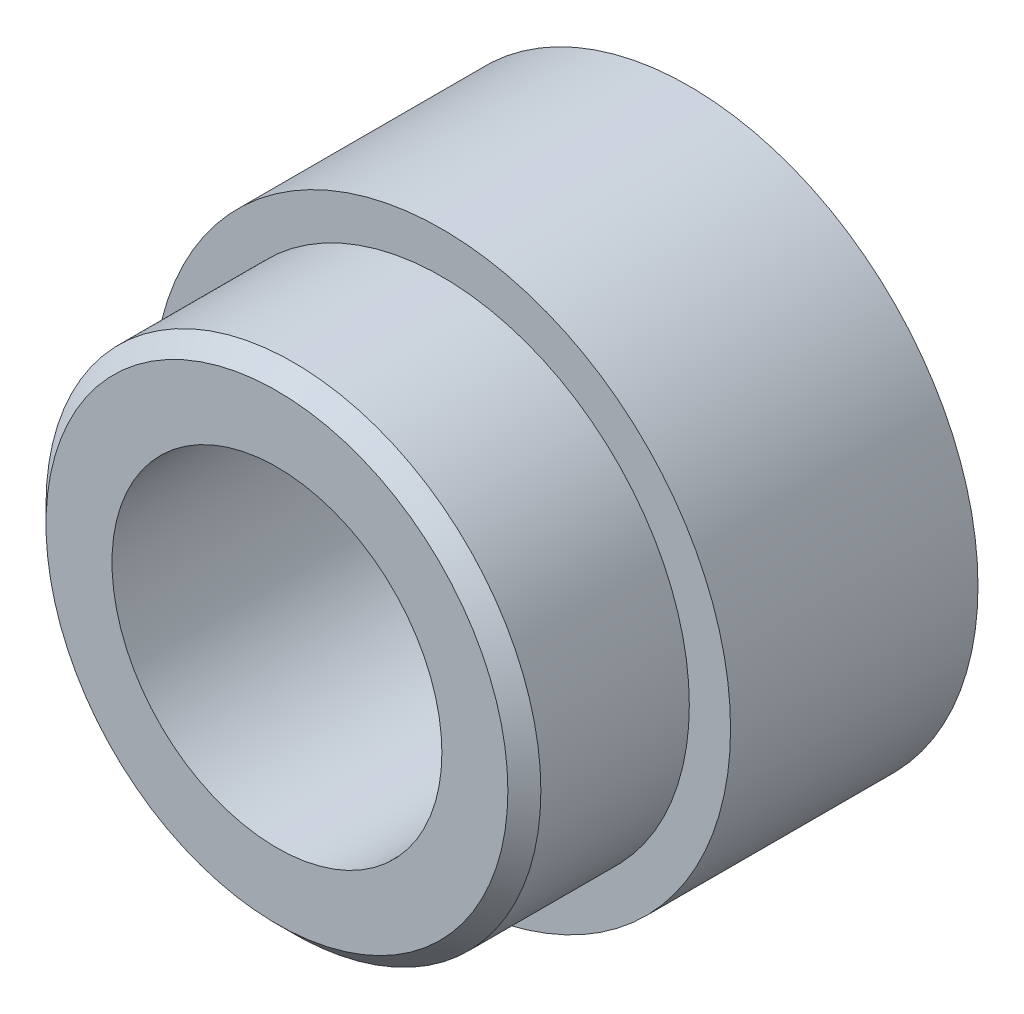
from build123d import *

# Parameters (mm, degrees)
SKETCH1_R           = 17.5
SKETCH1_R_2         = 10
BOSS_EXTRUDE1_DEPTH = 25
CUT_EXTRUDE1_START  = -10
SKETCH2_R           = 17.5
SKETCH2_R_2         = 15
CUT_EXTRUDE1_DEPTH  = 10
CHAMFER1_SIZE       = 1


with BuildPart() as part:
    # Sketch1 → Boss-Extrude1 (new body)
    with BuildSketch(Plane.XY):
        Circle(SKETCH1_R)
        Circle(SKETCH1_R_2, mode=Mode.SUBTRACT)
    extrude(amount=BOSS_EXTRUDE1_DEPTH)

    # Sketch2 → Cut-Extrude1 (cut)
    with BuildSketch(Plane.XY.offset(25).offset(CUT_EXTRUDE1_START)):
        Circle(SKETCH2_R)
        Circle(SKETCH2_R_2, mode=Mode.SUBTRACT)
    extrude(amount=CUT_EXTRUDE1_DEPTH, mode=Mode.SUBTRACT)

    # Chamfer1
    chamfer1_edges = [part.edges().sort_by_distance(p)[0] for p in [
        (-15, 0, 25),
    ]]
    chamfer(chamfer1_edges, length=CHAMFER1_SIZE)


solid = part.part
